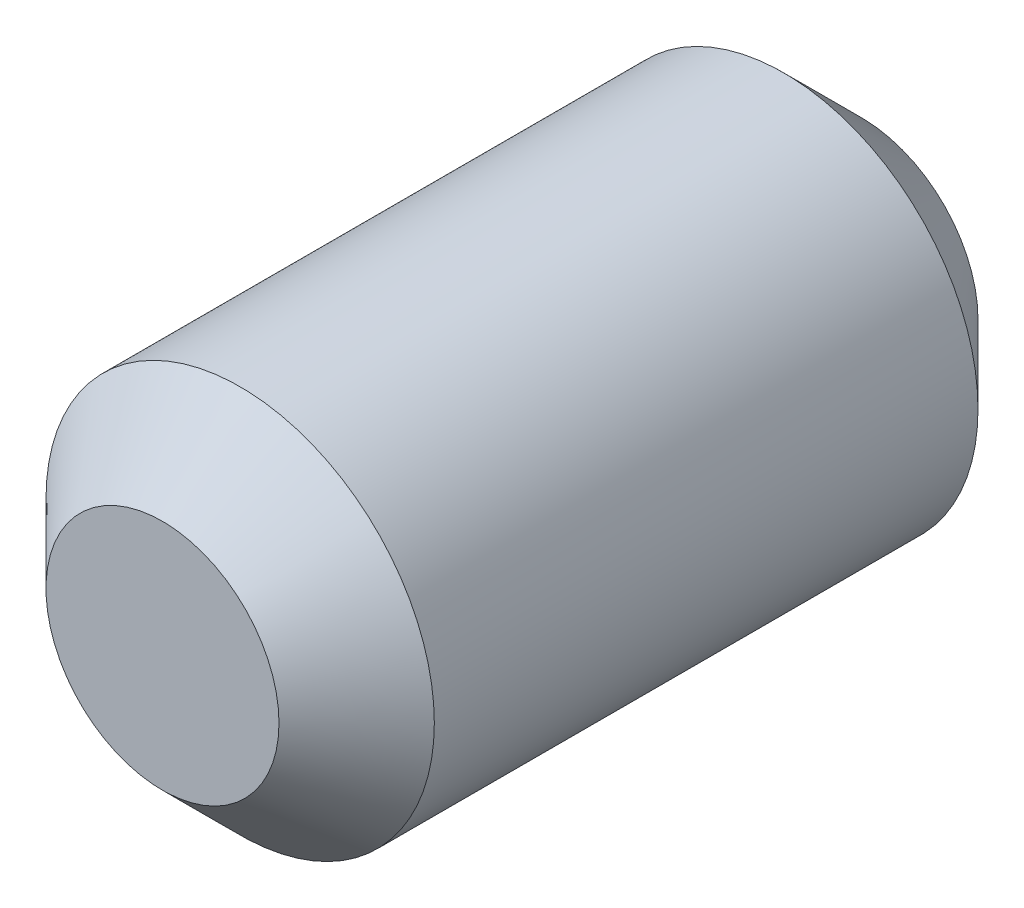
from build123d import *

# Parameters (mm, degrees)
SKETCH1_R           = 2.5
BOSS_EXTRUDE1_DEPTH = 9
CHAMFER1_SIZE       = 1


with BuildPart() as part:
    # Sketch1 → Boss-Extrude1 (new body)
    with BuildSketch(Plane.XY):
        Circle(SKETCH1_R)
    extrude(amount=BOSS_EXTRUDE1_DEPTH)

    # Chamfer1
    chamfer1_edges = [part.edges().sort_by_distance(p)[0] for p in [
        (-2.5, 0, 0),
        (-2.5, 0, 9),
    ]]
    chamfer(chamfer1_edges, length=CHAMFER1_SIZE)


solid = part.part
